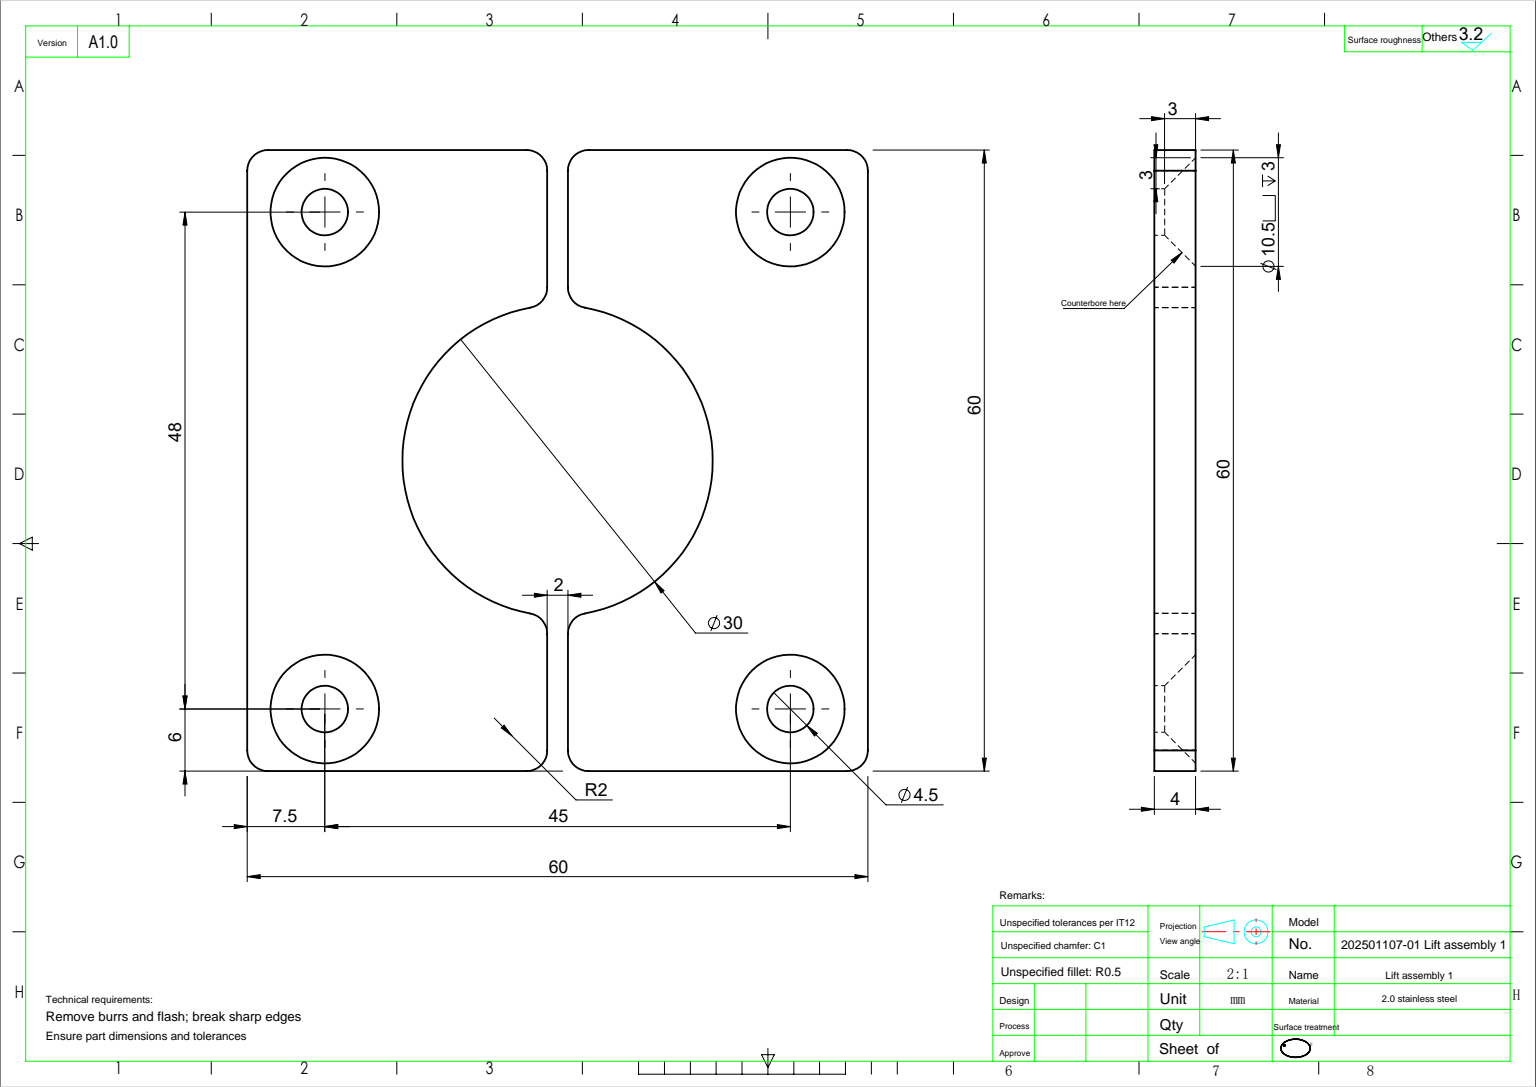
SolidWorks part; units mm, degrees
ref_plane "前视基准面" through (0, 0, 0) normal (0, 0, 1) x (1, 0, 0)
ref_plane "上视基准面" through (0, 0, 0) normal (0, 1, 0) x (1, 0, 0)
ref_plane "右视基准面" through (0, 0, 0) normal (1, 0, 0) x (0, 0, -1)
sketch "草图1" plane through (0, 0, 0) normal (0, 0, 1) x (1, 0, 0)
  line L1 (-30, 30) -> (30, 30)
  line L2 (-30, 30) -> (-30, -30)
  line L3 (-30, -30) -> (30, -30)
  line L4 (30, 30) -> (30, -30)
  line L5 (0, -30) -> (0, 30) construction
  line L6 (-30, 0) -> (30, 0) construction
  circle A1 centre (0, 0) radius 15
  point P0 (0, 0)
  dimension "D1" = 60
  dimension "D3" = 30
  dimension "D2" = 60
extrude "凸台-拉伸1" add sketch "草图1" along normal blind 4
sketch "草图2" plane through (0, 0, 4) normal (0, 0, 1) x (1, 0, 0)
  line L1 (-1, 36.8616) -> (1, 36.8616)
  line L2 (-1, 36.8616) -> (-1, -36.8616)
  line L3 (-1, -36.8616) -> (1, -36.8616)
  line L4 (1, 36.8616) -> (1, -36.8616)
  line L5 (0, -36.8616) -> (0, 36.8616) construction
  line L6 (-1, 0) -> (1, 0) construction
  point P0 (0, 0)
  dimension "D1" = 2
extrude "切除-拉伸1" cut sketch "草图2" against normal blind 20
sketch "草图3" plane through (0, 0, 4) normal (0, 0, 1) x (1, 0, 0)
  line L1 (-30, 30) -> (-30, -30) construction
  line L5 (1, -30) -> (30, -30) construction
  circle A0 centre (-22.5, 24) radius 2.25
  circle A1 centre (22.5, 24) radius 2.25
  circle A2 centre (-22.5, -24) radius 2.25
  circle A3 centre (22.5, -24) radius 2.25
  dimension "D1" = 4.5
  dimension "D2" = 48
  dimension "D3" = 45
  dimension "D4" = 7.5
  dimension "D5" = 6
extrude "切除-拉伸2" cut sketch "草图3" against normal blind 10
chamfer "倒角1" distance 3 angle 45 2 edges at (-20.25, -24, 4) (-20.25, 24, 4)
chamfer "倒角2" distance 3 angle 45 2 edges at (24.75, -24, 4) (24.75, 24, 4)
fillet "圆角1" radius 2 6 edges at (1, 30, 2) (1, -30, 2) (30, 30, 2) (30, -30, 2) (1, 14.9666, 2) (1, -14.9666, 2)
fillet "圆角2" radius 2 6 edges at (-30, 30, 2) (-30, -30, 2) (-1, 14.9666, 2) (-1, -14.9666, 2) (-1, 30, 2) (-1, -30, 2)
